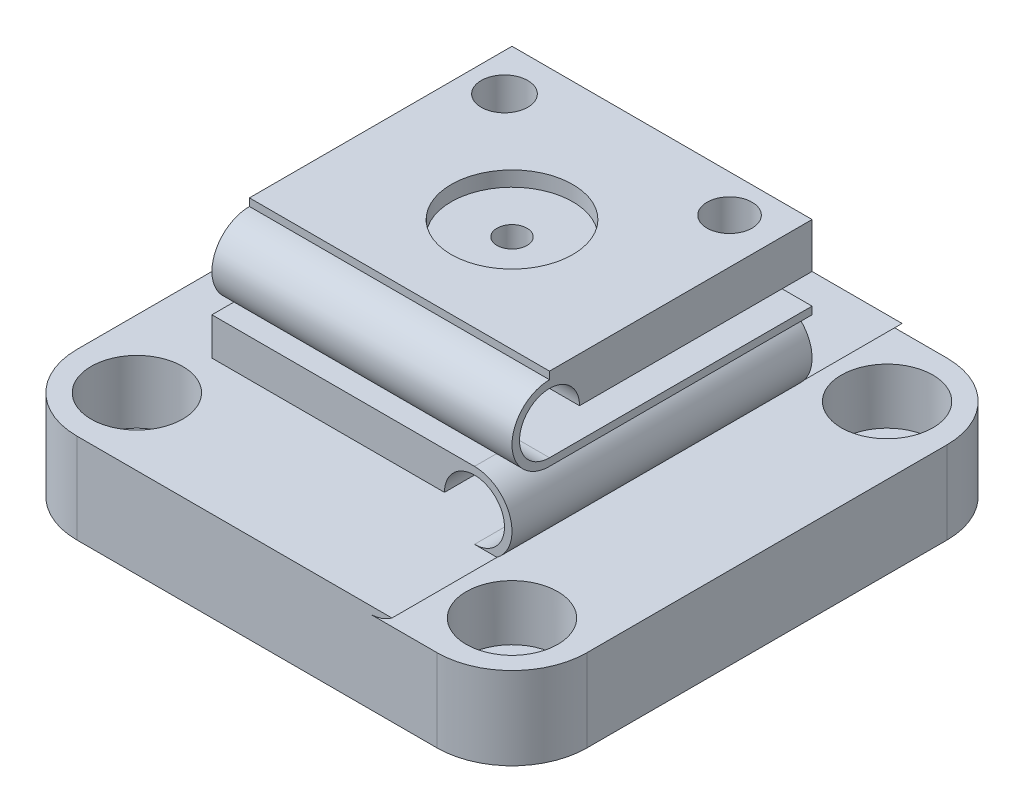
SolidWorks part; units mm, degrees
material "合金钢 (SS)"
ref_plane "Front Plane" through (0, 0, 0) normal (0, 0, 1) x (1, 0, 0)
ref_plane "Top Plane" through (0, 0, 0) normal (0, 1, 0) x (1, 0, 0)
ref_plane "Right Plane" through (0, 0, 0) normal (1, 0, 0) x (0, 0, -1)
sketch "Sketch1" plane through (0, 0, 0) normal (0, 1, 0) x (1, 0, 0)
  line L1 (-17, -17) -> (17, -17)
  line L2 (-17, -17) -> (-17, 17)
  line L3 (-17, 17) -> (17, 17)
  line L4 (17, -17) -> (17, 17)
  line L5 (-17, -17) -> (17, 17) construction
  line L6 (-17, 17) -> (17, -17) construction
  point P0 (0, 0)
  dimension "D1" = 34
  dimension "D2" = 34
extrude "Boss-Extrude1" add sketch "Sketch1" along normal blind 6
sketch "Sketch2" plane through (0, 6, 0) normal (0, 1, 0) x (1, 0, 0)
  line L1 (-12.5, -12.5) -> (12.5, -12.5) construction
  line L2 (-12.5, -12.5) -> (-12.5, 12.5) construction
  line L3 (-12.5, 12.5) -> (12.5, 12.5) construction
  line L4 (12.5, -12.5) -> (12.5, 12.5) construction
  line L5 (-12.5, -12.5) -> (12.5, 12.5) construction
  line L6 (-12.5, 12.5) -> (12.5, -12.5) construction
  circle A0 centre (-12.5, 12.5) radius 1.6
  circle A1 centre (12.5, 12.5) radius 1.6
  circle A2 centre (12.5, -12.5) radius 1.6
  circle A3 centre (-12.5, -12.5) radius 1.6
  point P0 (0, 0)
  dimension "D3" = 3.2
  dimension "D4" = 3.2
  dimension "D5" = 3.2
  dimension "D6" = 3.2
  dimension "D1" = 25
  dimension "D2" = 25
extrude "Cut-Extrude1" cut sketch "Sketch2" against normal blind 6
sketch "Sketch3" plane through (0, 6, 0) normal (0, 1, 0) x (1, 0, 0)
  circle A0 centre (-12.5, 12.5) radius 3.05
  circle A1 centre (12.5, 12.5) radius 3.05
  circle A2 centre (12.5, -12.5) radius 3.05
  circle A3 centre (-12.5, -12.5) radius 3.05
  dimension "D1" = 6.1
  dimension "D2" = 6.1
  dimension "D3" = 6.1
  dimension "D4" = 6.1
extrude "Cut-Extrude2" cut sketch "Sketch3" against normal blind 4.2
sketch "Sketch4" plane through (0, 6, 0) normal (0, 1, 0) x (1, 0, 0)
  line L1 (-10, -10) -> (10, -10)
  line L2 (-10, -10) -> (-10, 10)
  line L3 (-10, 10) -> (10, 10)
  line L4 (10, -10) -> (10, 10)
  line L5 (-10, -10) -> (10, 10) construction
  line L6 (-10, 10) -> (10, -10) construction
  point P0 (0, 0)
  dimension "D1" = 20
  dimension "D2" = 20
extrude "Boss-Extrude2" add sketch "Sketch4" along normal blind 10
sketch "Sketch5" plane through (0, 0, 17) normal (0, 0, 1) x (1, 0, 0)
  line L0 (10, 16) -> (10, 6) construction
  line L1 (-10, 6) -> (10, 6) construction
  line L2 (7.5, 10.5) -> (10, 10.5)
  line L3 (10, 10.5) -> (10, 6)
  line L5 (7.5, 6) -> (-10, 6)
  line L6 (5.5, 8) -> (-10, 8)
  line L7 (7.5, 6) -> (7.5, 5.5)
  line L9 (-10, 8) -> (-10, 6)
  line L10 (7.5, 5.5) -> (17, 5.5)
  line L11 (17, 6) -> (17, 0) construction
  line L12 (17, 5.5) -> (17, 6)
  line L13 (17, 6) -> (10, 6)
  arc A0 (7.5, 5.5) -> (7.5, 10.5) centre (7.5, 8) ccw
  arc A1 (7.5, 6) -> (5.5, 8) centre (7.5, 8) ccw
  line M2 (17, 0) -> (17, 6)
  line M3 (17, 6) -> (-17, 6)
  dimension "D1" = 5
  dimension "D2" = 4
  dimension "D3" = 2.5
  dimension "D4" = 2
extrude "Cut-Extrude4" cut sketch "Sketch5" against normal through all contours A1 L6 L9 M3 | A0 L3 L2 | A0 L3 M3 | A0 L10 M2 M3
sketch "Sketch6" plane through (-10, 0, 0) normal (-1, 0, 0) x (0, 0, 1)
  line L0 (10, 16) -> (10, 8) construction
  line L1 (-10, 16) -> (10, 16) construction
  line L2 (7.5, 10.5) -> (10, 10.5)
  line L3 (10, 10.5) -> (10, 15.5)
  line L4 (10, 15.5) -> (10, 16)
  line L5 (10, 16) -> (7.5, 16)
  line L6 (7.5, 16) -> (7.5, 15.5)
  line L7 (-10, 16) -> (-10, 8) construction
  line L8 (7.5, 13) -> (-10, 13)
  line L9 (7.5, 13) -> (7.5, 11)
  line L10 (7.5, 11) -> (-10, 11)
  line L11 (-10, 13) -> (-10, 11)
  circle A0 centre (7.5, 13) radius 2.5
  circle A1 centre (7.5, 13) radius 2
  line M1 (-10, 16) -> (-10, 8)
  line M3 (10, 8) -> (10, 16)
  line M4 (10, 16) -> (-10, 16)
  dimension "D1" = 5
  dimension "D2" = 4
  dimension "D3" = 2.5
  dimension "D4" = 3
extrude "Cut-Extrude5" cut sketch "Sketch6" against normal through all contours A0 L8 L10 M1 | A1 L8 A0 L10 | L8 A1 L9 | L9 A1 L8 | A0 L3 L6 M3 M4 | A0 L2 M3
sketch "Sketch7" plane through (0, 16, 0) normal (0, 1, 0) x (1, 0, 0)
  line L0 (9.5, 10) -> (5.5, 10) construction
  line L1 (-10, 10) -> (-10, -7.5) construction
  circle A0 centre (7, 7.5) radius 1.5
  dimension "D1" = 3
  dimension "D2" = 2.5
  dimension "D3" = 17
extrude "Cut-Extrude6" cut sketch "Sketch7" against normal blind 4
fillet "Fillet1" radius 5 4 edges at (-17, 3, -17) (-17, 3, 17) (17, 2.75, 17) (17, 2.75, -17)
sketch "Sketch8" plane through (0, 16, 0) normal (0, 1, 0) x (1, 0, 0)
  circle A0 centre (0, 0) radius 1
  dimension "D1" = 2
extrude "Cut-Extrude7" cut sketch "Sketch8" against normal blind 4
sketch "Sketch9" plane through (0, 16, 0) normal (0, 1, 0) x (1, 0, 0)
  circle A0 centre (0, 0) radius 4.05
  dimension "D1" = 8.1
extrude "Cut-Extrude8" cut sketch "Sketch9" against normal blind 1
sketch "Sketch10" plane through (0, 16, 0) normal (0, 1, 0) x (1, 0, 0)
  line L0 (-10, 10) -> (-10, -7.5) construction
  line L1 (10, 10) -> (-10, 10) construction
  circle A0 centre (-7.5, 7) radius 1.55
  dimension "D1" = 3.1
  dimension "D2" = 2.5
  dimension "D3" = 3
extrude "Cut-Extrude9" cut sketch "Sketch10" against normal blind 9
